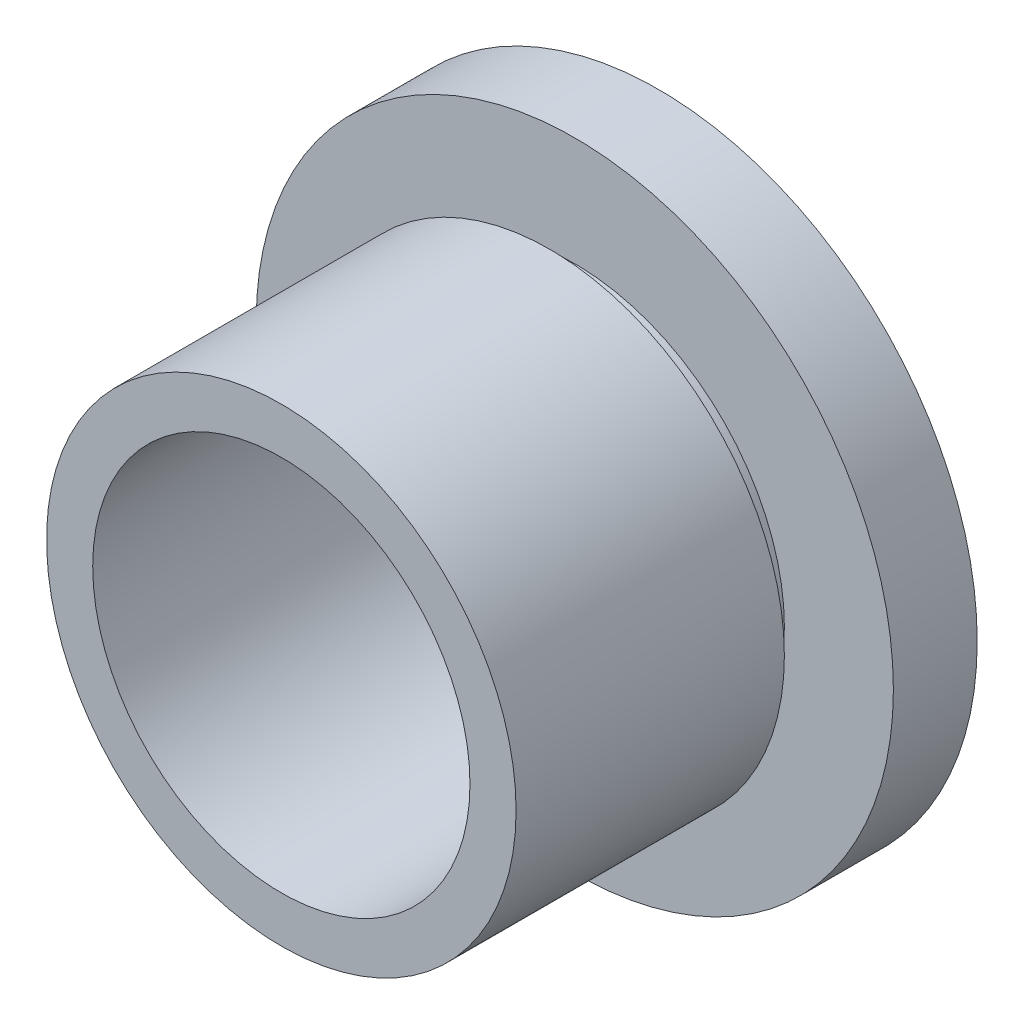
from build123d import *


with BuildPart() as part:
    # Sketch1 → Revolve1 (revolve)
    with BuildSketch(Plane(origin=(0, 0, 0), x_dir=(0, 0, -1), z_dir=(1, 0, 0)), mode=Mode.PRIVATE) as revolve1_sk:
        Polygon((0, 22.5), (0, 28), (32, 28), (32, 25), (35, 25), (35, 38), (45, 38), (45, 17.5), (35, 17.5), (35, 22.5), align=None)
    revolve(revolve1_sk.sketch.rotate(Axis((0, 0, 12.011308803), (0, 0, -1)), 90), axis=Axis((0, 0, 12.011308803), (0, 0, -1)))


solid = part.part
